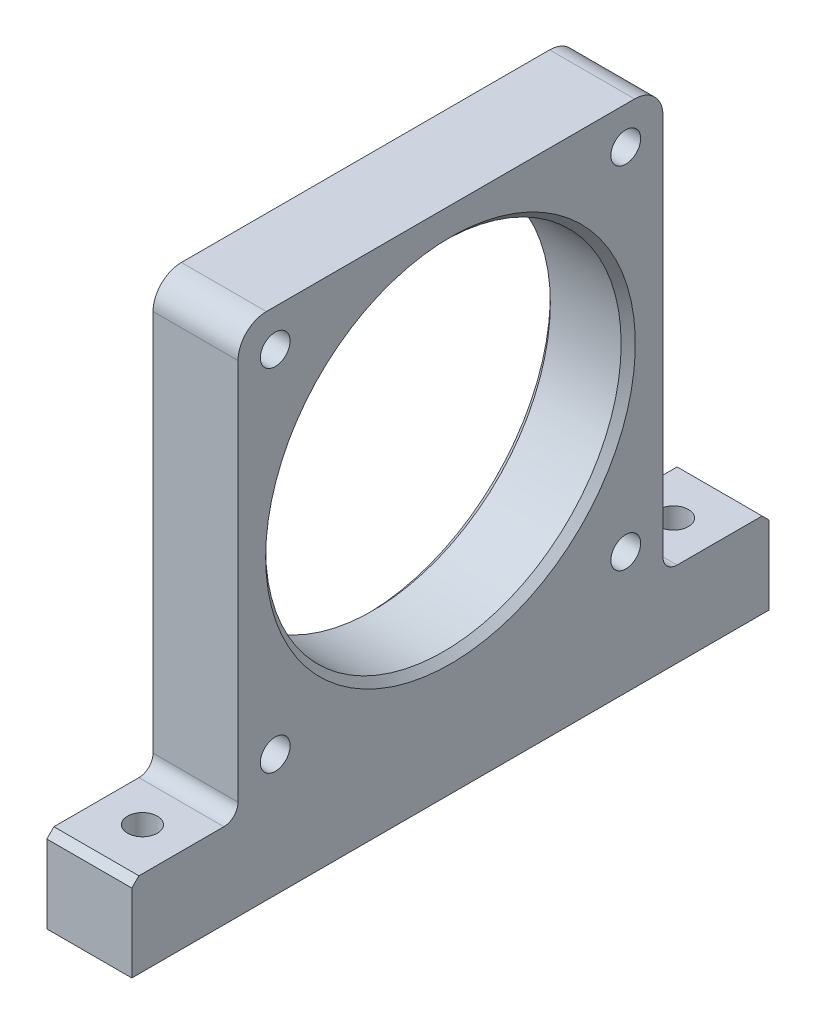
SolidWorks part; units mm, degrees
material "S45C"
ref_plane "Front Plane" through (0, 0, 0) normal (0, 0, 1) x (1, 0, 0)
ref_plane "Top Plane" through (0, 0, 0) normal (0, 1, 0) x (1, 0, 0)
ref_plane "Right Plane" through (0, 0, 0) normal (1, 0, 0) x (0, 0, -1)
sketch "Sketch1" plane through (0, 0, 0) normal (1, 0, 0) x (0, 0, -1)
  line L0 (0, 86.407) -> (0, -32.5375) construction
  line L1 (-45, 0) -> (45, 0)
  line L2 (-45, 0) -> (-45, 12)
  line L3 (-30, 72) -> (30, 72)
  line L4 (45, 0) -> (45, 12)
  line L5 (30, 42) -> (-30, 42) construction
  line L7 (45, 12) -> (30, 12)
  line L8 (30, 72) -> (30, 12)
  line L11 (-45, 12) -> (-30, 12)
  line L12 (-30, 72) -> (-30, 12)
  circle A0 centre (0, 42) radius 25.1
  dimension "D5" = 50.2
  dimension "D1" = 60
  dimension "D2" = 60
  dimension "D3" = 90
  dimension "D4" = 12
extrude "Boss-Extrude1" add sketch "Sketch1" along normal mid plane 12
fillet "Fillet1" radius 4 2 edges at (0, 72, 30) (0, 72, -30)
fillet "Fillet2" radius 2 2 edges at (0, 12, 30) (0, 12, -30)
chamfer "Chamfer1" distance 1 angle 45 2 edges at (0, 12, 45) (0, 12, -45)
hole_wizard "M5 Tapped Hole2" positions "Sketch4" profile "Sketch2" tap size "M5" standard "Gb" end condition through all
sketch "Sketch4" plane through (0, 12, 0) normal (0, 1, 0) x (1, 0, 0)
  line L0 (-13.6046, 0) -> (16.6493, 0) construction
  point P0 (0, -37.5)
  point P2 (0, 37.5)
  dimension "D1" = 75
sketch "Sketch2" plane through (0, 12, 37.5) normal (1, 0, 0) x (0, 0, 1)
  line L0 (0, 0) -> (0, 12)
  line L1 (0, 12) -> (2.1, 12)
  line L2 (2.1, 12) -> (2.1, 0)
  line L5 (2.1, 0) -> (0, 0)
  line L11 (0, -6.35) -> (0, 107.95) construction
  dimension "通孔螺纹孔钻头直径" = 4.2
  dimension "通孔螺纹孔钻头深度" = 12
cosmetic thread "Cosmetic Thread5" parameters "D2"=5
cosmetic thread "Cosmetic Thread6" parameters "D2"=5
hole_wizard "M5 Tapped Hole1" positions "Sketch6" profile "Sketch5" tap size "M5" standard "Gb"
sketch "Sketch6" plane through (6, 0, 0) normal (1, 0, 0) x (0, 0, -1)
  line L0 (0, 42) -> (24.7487, 66.7487) construction
  line L3 (0, 42) -> (-24.7487, 66.7487) construction
  line L6 (0, 42) -> (-24.7487, 17.2513) construction
  line L9 (0, 42) -> (24.7487, 17.2513) construction
  line L12 (0, 42) -> (37.9934, 42) construction
  circle A0 centre (0, 42) radius 35 construction
  point P0 (-24.7487, 66.7487)
  point P2 (24.7487, 66.7487)
  point P4 (24.7487, 17.2513)
  point P6 (-24.7487, 17.2513)
  dimension "D1" = 70
  dimension "D2" = 45
  dimension "D3" = 45
sketch "Sketch5" plane through (6, 66.7487, 24.7487) normal (0, 1, 0) x (0, 0, -1)
  line L0 (0, 0) -> (0, 15.2618)
  line L1 (0, 15.2618) -> (2.1, 14)
  line L2 (2.1, 14) -> (2.1, 0)
  line L5 (2.1, 0) -> (0, 0)
  line L10 (0, 15.2618) -> (-2.1, 14) construction
  line L11 (0, -6.35) -> (0, 107.95) construction
  dimension "螺纹孔钻头直径" = 4.2
  dimension "螺纹孔钻头深度" = 14
  dimension "导头角度" = 118
cosmetic thread "Cosmetic Thread1" parameters "D1"=10, "D2"=5
cosmetic thread "Cosmetic Thread2" parameters "D1"=10, "D2"=5
cosmetic thread "Cosmetic Thread3" parameters "D1"=10, "D2"=5
cosmetic thread "Cosmetic Thread4" parameters "D1"=10, "D2"=5
chamfer "Chamfer2" distance 1 angle 45 2 edges at (-6, 42, -25.1) (6, 42, -25.1)
